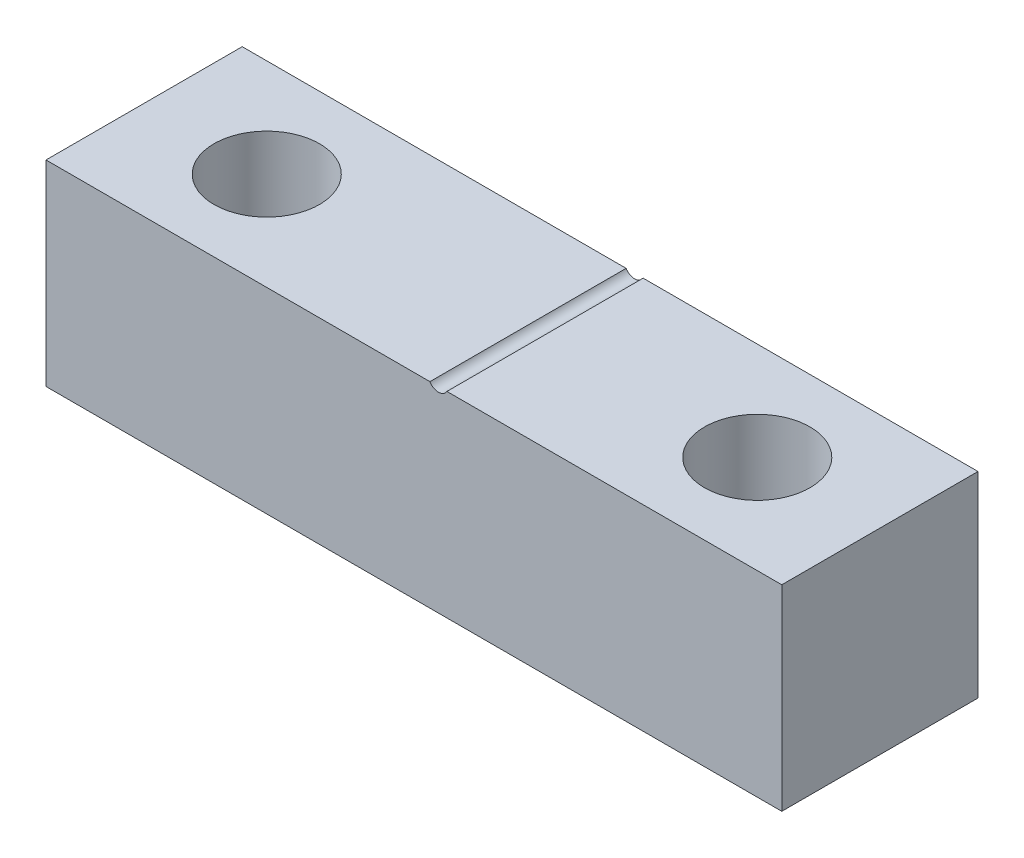
SolidWorks part; units mm, degrees
ref_plane "前视基准面" through (0, 0, 0) normal (0, 0, 1) x (1, 0, 0)
ref_plane "上视基准面" through (0, 0, 0) normal (0, 1, 0) x (1, 0, 0)
ref_plane "右视基准面" through (0, 0, 0) normal (1, 0, 0) x (0, 0, -1)
sketch "草图1" plane through (0, 0, 0) normal (0, 0, 1) x (1, 0, 0)
  line L1 (-12.9071, 2.7509) -> (17.0929, 2.7509)
  line L2 (-12.9071, 2.7509) -> (-12.9071, -5.2491)
  line L3 (-12.9071, -5.2491) -> (17.0929, -5.2491)
  line L4 (17.0929, 2.7509) -> (17.0929, -5.2491)
  dimension "D1" = 8
  dimension "D2" = 30
extrude "凸台-拉伸1" add sketch "草图1" along normal blind 8
sketch "草图2" plane through (0, 2.7509, 0) normal (0, 1, 0) x (1, 0, 0)
  line L0 (17.0929, 0) -> (-12.9071, 0) construction
  line L1 (-12.9071, -8) -> (-12.9071, 0) construction
  line L2 (17.0929, -8) -> (17.0929, 0) construction
  circle A0 centre (-7.9071, -4) radius 2.15
  circle A1 centre (12.0929, -4) radius 2.15
  dimension "D5" = 4.3
  dimension "D6" = 4.3
  dimension "D1" = 4
  dimension "D2" = 5
  dimension "D3" = 4
  dimension "D4" = 5
extrude "切除-拉伸1" cut sketch "草图2" against normal through all
sketch "草图3" plane through (0, 0, 8) normal (0, 0, 1) x (1, 0, 0)
  line L1 (17.0929, 2.7509) -> (-12.9071, 2.7509) construction
  line L2 (17.0929, -5.2491) -> (17.0929, 2.7509) construction
  line L3 (2.7465, 2.7509) -> (3.4393, 2.7509)
  arc A0 (2.7465, 2.7509) -> (3.4393, 2.7509) centre (3.0929, 2.9509) ccw
  dimension "D3" = 0.8
  dimension "D1" = 0.2
  dimension "D2" = 14
extrude "切除-拉伸2" cut sketch "草图3" against normal through all
